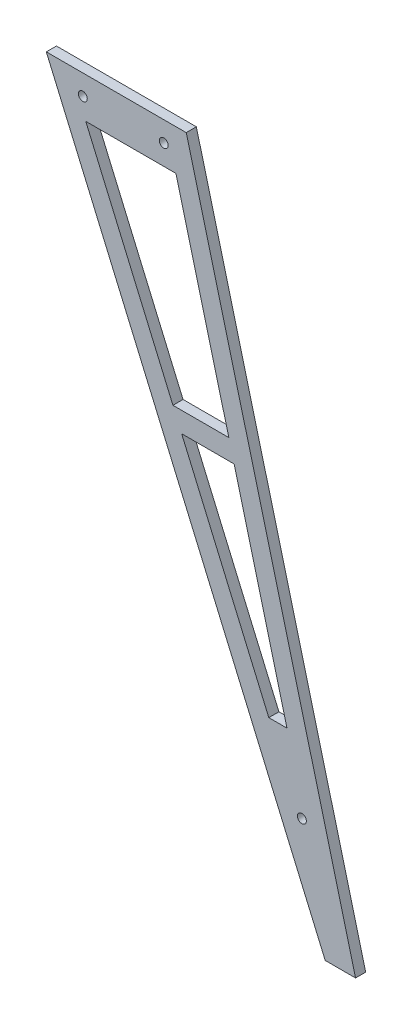
SolidWorks part; units mm, degrees
ref_plane "前视基准面" through (0, 0, 0) normal (0, 0, 1) x (1, 0, 0)
ref_plane "上视基准面" through (0, 0, 0) normal (0, 1, 0) x (1, 0, 0)
ref_plane "右视基准面" through (0, 0, 0) normal (1, 0, 0) x (0, 0, -1)
sketch "草图1" plane through (0, 0, 0) normal (0, 0, 1) x (1, 0, 0)
  line L0 (0, 0) -> (8, 0)
  line L1 (8, 0) -> (50, -240)
  line L2 (50, -240) -> (170, -338)
  line L3 (170, -338) -> (255, -663)
  line L4 (255, -663) -> (240, -663)
  line L5 (240, -663) -> (100, -338)
  line L6 (100, -338) -> (0, -240)
  line L8 (0, -240) -> (0, -113)
  line L9 (0, -113) -> (5, -113)
  line L10 (5, -113) -> (5, -63)
  line L11 (5, -63) -> (0, -63)
  line L12 (0, -63) -> (0, 0)
  line L13 (100, -338) -> (170, -338) construction
  line L14 (50, -240) -> (0, -240) construction
  line L15 (102.1538, -343) -> (171.3077, -343)
  dimension "D1" = 8
  dimension "D2" = 63
  dimension "D3" = 5
  dimension "D4" = 50
  dimension "D5" = 15
  dimension "D6" = 255
  dimension "D7" = 50
  dimension "D8" = 98
  dimension "D9" = 240
  dimension "D10" = 325
  dimension "D11" = 170
  dimension "D12" = 70
  dimension "D13" = 5
extrude "凸台-拉伸1" add sketch "草图1" along normal mid plane 5 contours L15 L5 L4 L3
sketch "草图3" plane through (0, 0, 2.5) normal (0, 0, 1) x (1, 0, 0)
  line L0 (135, -338) -> (247.5, -663) construction
  line L1 (100, -338) -> (170, -338) construction
  line L2 (255, -663) -> (240, -663) construction
  line L3 (120.1923, -353) -> (140.1923, -353) construction
  line L4 (140.1923, -353) -> (160.1923, -353) construction
  circle A0 centre (120.1923, -353) radius 2.2
  circle A1 centre (160.1923, -353) radius 2.2
  dimension "D3" = 4.4
  dimension "D1" = 15
  dimension "D2" = 20
extrude "切除-拉伸1" cut sketch "草图3" against normal blind 10
sketch "草图4" plane through (0, 0, 2.5) normal (0, 0, 1) x (1, 0, 0)
  line L4 (121.6576, -363) -> (166.2021, -363)
  line L5 (164.7345, -463) -> (235.1485, -463)
  line L6 (161.826, -473) -> (235.4376, -473)
  line L7 (197.7402, -573) -> (259.0602, -573)
  line L8 (163.5867, -353) -> (117.3499, -353)
  line L9 (117.3499, -353) -> (235.0436, -626.2176)
  line L10 (235.0436, -626.2176) -> (163.5867, -353)
  line L11 (163.5867, -353) -> (117.3499, -353)
  line L12 (117.3499, -353) -> (235.0436, -626.2176)
  line L13 (235.0436, -626.2176) -> (163.5867, -353)
  dimension "D2" = 100
  dimension "D3" = 10
  dimension "D4" = 100
  dimension "D5" = 10
  dimension "D1" = 10
extrude "切除-拉伸2" cut sketch "草图4" against normal blind 10 contours L5 L13 L4 L12 | L7 L13 L6 L12
sketch "草图5" plane through (0, 0, 2.5) normal (0, 0, 1) x (1, 0, 0)
  line L0 (228.4615, -608) -> (247.5, -663) construction
  line L1 (255, -663) -> (240, -663) construction
  line L2 (135, -338) -> (228.4615, -608) construction
  line L3 (100, -338) -> (170, -338) construction
  circle A0 centre (228.4615, -608) radius 2.2
  dimension "D1" = 55
  dimension "D2" = 4.4
extrude "切除-拉伸3" cut sketch "草图5" against normal blind 10
